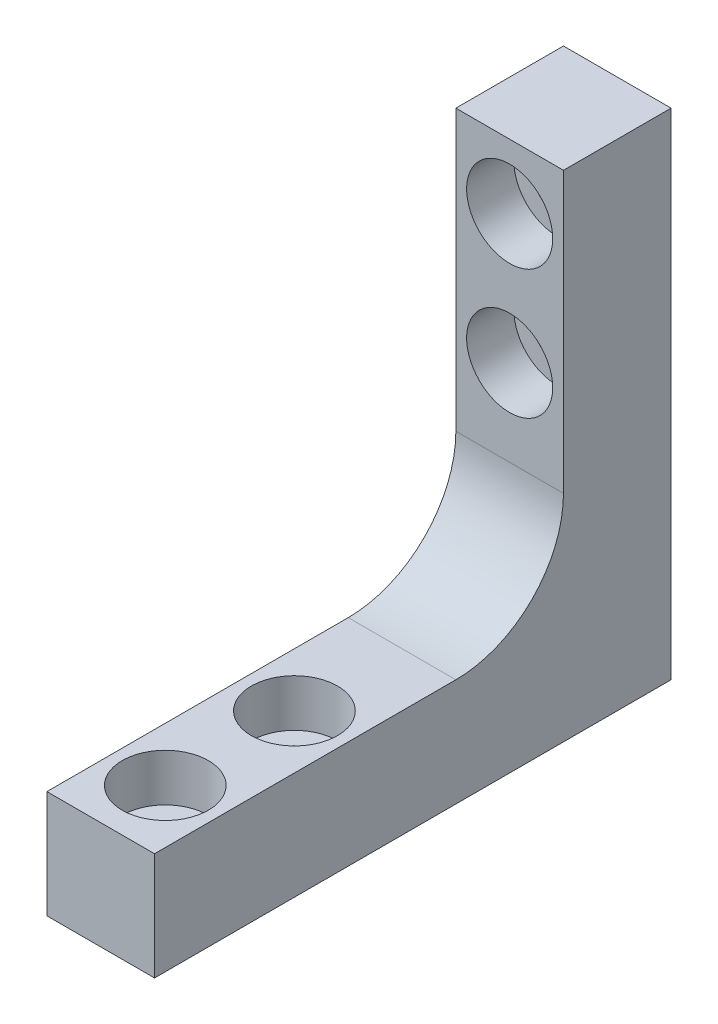
from build123d import *

# Parameters (mm, degrees)
SKETCH1_W                                           = 48
SKETCH1_H                                           = 46
BOSS_EXTRUDE1_DEPTH                                 = 5
SKETCH2_W                                           = 38
SKETCH2_H                                           = 36
CUT_EXTRUDE1_DEPTH                                  = 35.713109915
FILLET1_R                                           = 10
CBORE_FOR_M4_HEX_SOCKET_HEAD_CAP_SCREW1_D           = 4.5
CBORE_FOR_M4_HEX_SOCKET_HEAD_CAP_SCREW1_CBORE_D     = 8
CBORE_FOR_M4_HEX_SOCKET_HEAD_CAP_SCREW1_CBORE_DEPTH = 4.4
CBORE_FOR_M4_HEX_SOCKET_HEAD_CAP_SCREW2_D           = 4.5
CBORE_FOR_M4_HEX_SOCKET_HEAD_CAP_SCREW2_CBORE_D     = 8
CBORE_FOR_M4_HEX_SOCKET_HEAD_CAP_SCREW2_CBORE_DEPTH = 4.4


with BuildPart() as part:
    # Sketch1 → Boss-Extrude1 (new, symmetric)
    with BuildSketch(Plane(origin=(0, 0, 0), x_dir=(0, 0, -1), z_dir=(1, 0, 0))):
        Rectangle(SKETCH1_W, SKETCH1_H)
    extrude(amount=BOSS_EXTRUDE1_DEPTH, both=True)

    # Sketch2 → Cut-Extrude1 (cut, through all)
    with BuildSketch(Plane(origin=(5, 0, 0), x_dir=(0, 0, -1), z_dir=(1, 0, 0))):
        with Locations((-5, 5)):
            Rectangle(SKETCH2_W, SKETCH2_H)
    extrude(amount=-CUT_EXTRUDE1_DEPTH, mode=Mode.SUBTRACT)

    # Fillet1
    fillet1_edges = [part.edges().sort_by_distance(p)[0] for p in [
        (0, -13, -14),
    ]]
    fillet(fillet1_edges, radius=FILLET1_R)

    # CBORE for M4 Hex Socket Head Cap Screw1 (through all)
    with Locations(Plane(origin=(0, -13, 0), x_dir=(1, 0, 0), z_dir=(0, 1, 0))):
        with Locations((0, -18), (0, -6)):
            CounterBoreHole(CBORE_FOR_M4_HEX_SOCKET_HEAD_CAP_SCREW1_D / 2, CBORE_FOR_M4_HEX_SOCKET_HEAD_CAP_SCREW1_CBORE_D / 2, CBORE_FOR_M4_HEX_SOCKET_HEAD_CAP_SCREW1_CBORE_DEPTH)

    # CBORE for M4 Hex Socket Head Cap Screw2 (through all)
    with Locations(Plane.XY.offset(-14)):
        with Locations((0, 17), (0, 5)):
            CounterBoreHole(CBORE_FOR_M4_HEX_SOCKET_HEAD_CAP_SCREW2_D / 2, CBORE_FOR_M4_HEX_SOCKET_HEAD_CAP_SCREW2_CBORE_D / 2, CBORE_FOR_M4_HEX_SOCKET_HEAD_CAP_SCREW2_CBORE_DEPTH)


solid = part.part
